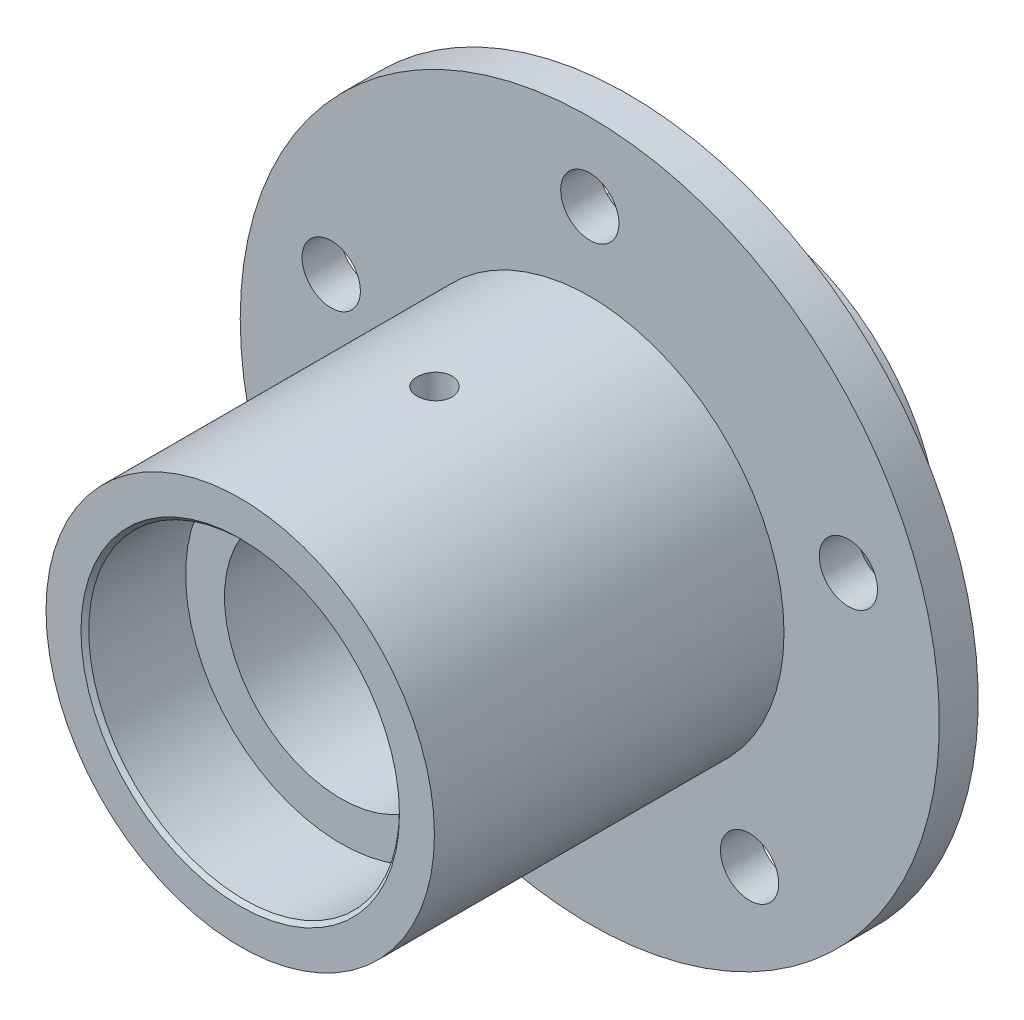
SolidWorks part; units mm, degrees
material "普通碳钢"
ref_plane "前视基准面" through (0, 0, 0) normal (0, 0, 1) x (1, 0, 0)
ref_plane "上视基准面" through (0, 0, 0) normal (0, 1, 0) x (1, 0, 0)
ref_plane "右视基准面" through (0, 0, 0) normal (1, 0, 0) x (0, 0, -1)
sketch "草图1" plane through (0, 0, 0) normal (0, 0, 1) x (1, 0, 0)
  circle A0 centre (0, 0) radius 50
  dimension "D1" = 100
extrude "凸台-拉伸1" add sketch "草图1" along normal blind 120 and the other way blind 10
sketch "草图2" plane through (0, 0, 120) normal (0, 0, 1) x (1, 0, 0)
  circle A0 centre (0, 0) radius 30
  dimension "D1" = 60
extrude "切除-拉伸1" cut sketch "草图2" against normal blind 120
sketch "草图3" plane through (0, 0, 120) normal (0, 0, 1) x (1, 0, 0)
  circle A0 centre (0, 0) radius 40
  dimension "D1" = 80
extrude "切除-拉伸2" cut sketch "草图3" against normal blind 25.95
sketch "草图4" plane through (0, 0, -10) normal (0, 0, -1) x (-1, 0, 0)
  circle A0 centre (0, 0) radius 40
extrude "切除-拉伸3" cut sketch "草图4" against normal blind 35.95
ref_plane "基准面2" through (0, 0, 60) normal (0, 0, 1) x (1, 0, 0)
ref_plane "基准面3" through (0, 0, 20) normal (0, 0, -1) x (-1, 0, 0)
sketch "草图6" plane through (0, 0, 20) normal (0, 0, -1) x (-1, 0, 0)
  circle A0 centre (0, 0) radius 50
  circle A1 centre (0, 0) radius 90
  dimension "D1" = 180
extrude "凸台-拉伸2" add sketch "草图6" against normal blind 10 separate body
ref_plane "基准面4" through (0, 50, 0) normal (0, 1, 0) x (1, 0, 0)
sketch "草图7" plane through (0, 50, 0) normal (0, 1, 0) x (1, 0, 0)
  line L0 (0, 0) -> (0, -120) construction
  line L1 (-50, -120) -> (50, -120) construction
  circle A0 centre (0, -70) radius 2.5
  dimension "D1" = 50
  dimension "D2" = 5
extrude "切除-拉伸5" cut sketch "草图7" against normal blind 30
hole_wizard "M10x1.0 螺纹孔1" positions "草图9" profile "草图8" tap size "M10x1.0" standard "GB"
sketch "草图9" plane through (0, 50, 0) normal (0, 1, 0) x (1, 0, 0)
  point P0 (0, -70)
sketch "草图8" plane through (0, 50, 70) normal (1, 0, 0) x (0, 0, 1)
  line L0 (0, 0) -> (0, 11)
  line L1 (0, 11) -> (4.5, 8.2961)
  line L2 (4.5, 8.2961) -> (4.5, 0)
  line L5 (4.5, 0) -> (0, 0)
  line L10 (0, 11) -> (-4.5, 8.2961) construction
  line L11 (0, -6.35) -> (0, 107.95) construction
  dimension "螺纹孔钻头直径" = 9
  dimension "螺纹孔钻头深度" = 11
  dimension "导头角度" = 118
cosmetic thread "孔螺蚊线1" parameters "D1"=6, "D2"=10
sketch "草图11" plane through (0, 0, 20) normal (0, 0, -1) x (-1, 0, 0)
  circle A0 centre (0, 0) radius 70 construction
  circle A1 centre (0, 70) radius 7.5
  circle A2 centre (66.574, 21.6312) radius 7.5
  circle A3 centre (41.145, -56.6312) radius 7.5
  circle A4 centre (-41.145, -56.6312) radius 7.5
  circle A5 centre (-66.574, 21.6312) radius 7.5
  dimension "D1" = 5
extrude "切除-拉伸6" cut sketch "草图11" against normal blind 10
ref_plane "基准面5" through (0, 0, 5.3) normal (0, 0, -1) x (-1, 0, 0)
sketch "草图12" plane through (0, 0, 5.3) normal (0, 0, -1) x (-1, 0, 0)
  circle A0 centre (0, 0) radius 40
  circle A1 centre (0, 0) radius 41.75
  dimension "D1" = 80
  dimension "D2" = 83.5
extrude "切除-拉伸7" cut sketch "草图12" against normal blind 2.7
sketch "草图13" plane through (0, 0, -10) normal (0, 0, -1) x (-1, 0, 0)
  circle A0 centre (0, 0) radius 45 construction
  circle A1 centre (0, 45) radius 3 construction
  circle A2 centre (38.9711, 22.5) radius 3 construction
  circle A3 centre (38.9711, -22.5) radius 3 construction
  circle A4 centre (0, -45) radius 3 construction
  circle A5 centre (-38.9711, -22.5) radius 3 construction
  circle A6 centre (-38.9711, 22.5) radius 3 construction
  dimension "D1" = 90
  dimension "D2" = 6
  dimension "D3" = 6
hole_wizard "M6 螺纹孔1" positions "草图16" profile "草图17" tap size "M6" standard "GB"
sketch "草图16" plane through (0, 0, -10) normal (0, 0, -1) x (-1, 0, 0)
  point P0 (0, 45)
  point P3 (38.9711, 22.5)
  point P6 (38.9711, -22.5)
  point P9 (0, -45)
  point P12 (-38.9711, -22.5)
  point P15 (-38.9711, 22.5)
sketch "草图17" plane through (0, 45, -10) normal (1, 0, 0) x (0, 1, 0)
  line L0 (0, 0) -> (0, 16.5022)
  line L1 (0, 16.5022) -> (2.5, 15)
  line L2 (2.5, 15) -> (2.5, 0)
  line L5 (2.5, 0) -> (0, 0)
  line L10 (0, 16.5022) -> (-2.5, 15) construction
  line L11 (0, -6.35) -> (0, 107.95) construction
  dimension "螺纹孔钻头直径" = 5
  dimension "螺纹孔钻头深度" = 15
  dimension "导头角度" = 118
cosmetic thread "孔螺蚊线2" parameters "D1"=10, "D2"=6
cosmetic thread "孔螺蚊线3" parameters "D1"=10, "D2"=6
cosmetic thread "孔螺蚊线4" parameters "D1"=10, "D2"=6
cosmetic thread "孔螺蚊线5" parameters "D1"=10, "D2"=6
cosmetic thread "孔螺蚊线6" parameters "D1"=10, "D2"=6
cosmetic thread "孔螺蚊线7" parameters "D1"=10, "D2"=6
chamfer "倒角1" distance 1 angle 45 2 edges at (40, 0, 120) (-40, 0, -10)
